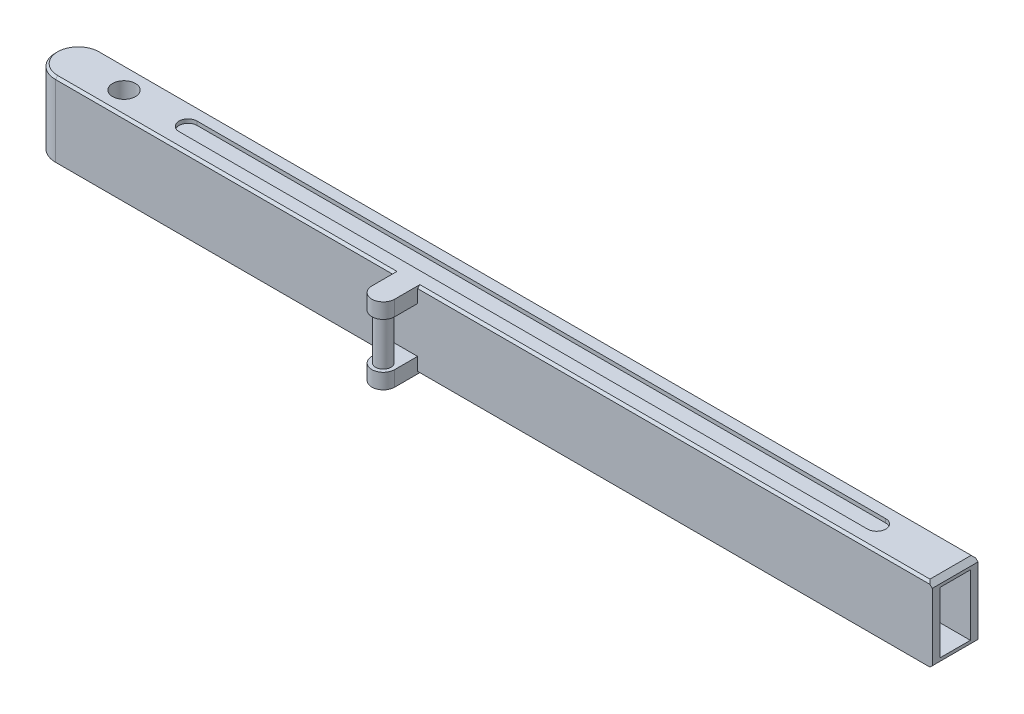
SolidWorks part; units mm, degrees
ref_plane "Front Plane" through (0, 0, 0) normal (0, 0, 1) x (1, 0, 0)
ref_plane "Top Plane" through (0, 0, 0) normal (0, 1, 0) x (1, 0, 0)
ref_plane "Right Plane" through (0, 0, 0) normal (1, 0, 0) x (0, 0, -1)
sketch "Sketch1" plane through (0, 0, 0) normal (0, 1, 0) x (1, 0, 0)
  line L0 (0, 0) -> (11500, 0)
  line L1 (11500, 0) -> (11500, 600)
  line L3 (0, 600) -> (694.445, 600)
  line L4 (11500, 300) -> (385.2625, 300) construction
  line L5 (11500, 600) -> (694.445, 600)
  arc A0 (0, 0) -> (0, 600) centre (0, 300) cw
  circle A2 centre (600, 300) radius 150
  dimension "D5" = 300
  dimension "D7" = 300
  dimension "D1" = 11500
  dimension "D2" = 600
  dimension "D3" = 90
  dimension "D8" = 10900
extrude "Boss-Extrude1" add sketch "Sketch1" along normal blind 1000
ref_plane "Plane1" through (0, 500, 0) normal (0, 1, 0) x (1, 0, 0)
sketch "Sketch3" plane through (0, 1000, 0) normal (0, 1, 0) x (1, 0, 0)
  line L0 (4600, 203.2624) -> (4600, -300) construction
  line L1 (4750, 203.2624) -> (4750, -300)
  line L2 (4450, 203.2624) -> (4450, -300)
  line L3 (-55, 0) -> (55, 0) construction
  arc A0 (4750, 203.2624) -> (4450, 203.2624) centre (4600, 203.2624) ccw
  arc A1 (4450, -300) -> (4750, -300) centre (4600, -300) ccw
  circle A2 centre (600, 300) radius 150 construction
  point P2 (4600, -48.3688)
  dimension "D1" = 150
  dimension "D3" = 4000
  dimension "D2" = 300
extrude "Boss-Extrude2" add sketch "Sketch3" against normal blind 200
mirror "Mirror1" about plane through (0, 500, 0) normal (0, 1, 0) of "Boss-Extrude2"
sketch "Sketch4" plane through (0, 800, 0) normal (0, -1, 0) x (1, 0, 0)
  circle A0 centre (4600, 300) radius 100
  dimension "D1" = 200
extrude "Boss-Extrude3" add sketch "Sketch4" along normal blind 700
sketch "Sketch5" plane through (11500, 0, 0) normal (1, 0, 0) x (0, 0, -1)
  line L0 (0, 55) -> (0, -55) construction
  line L1 (100, 900) -> (500, 900)
  line L2 (100, 900) -> (100, 100)
  line L3 (100, 100) -> (500, 100)
  line L4 (500, 900) -> (500, 100)
  line L5 (55, 0) -> (-55, 0) construction
  dimension "D1" = 400
  dimension "D2" = 100
  dimension "D3" = 800
  dimension "D4" = 100
extrude "Cut-Extrude1" cut sketch "Sketch5" against normal blind 10000
sketch "Sketch6" plane through (0, 0, 0) normal (0, -1, 0) x (1, 0, 0)
  line L0 (1432.066, -307.8009) -> (10462.7964, -307.8009) construction
  line L1 (1432.066, -188.6831) -> (10462.7964, -188.6831)
  line L2 (1432.066, -426.9188) -> (10462.7964, -426.9188)
  arc A0 (1432.066, -188.6831) -> (1432.066, -426.9188) centre (1432.066, -307.8009) ccw
  arc A1 (10462.7964, -426.9188) -> (10462.7964, -188.6831) centre (10462.7964, -307.8009) ccw
  point P2 (5947.4312, -307.8009)
extrude "Cut-Extrude2" cut sketch "Sketch6" against normal blind 50
mirror "Mirror2" about plane through (0, 500, 0) normal (0, 1, 0) of "Cut-Extrude2"
chamfer "Chamfer1" distance 30 angle 45 8 edges at (5750, 0, -600) (5750, 1000, -600) (-300, 0, -300) (-300, 1000, -300) (2225, 1000, 0) (2225, 0, 0) (8125, 0, 0) (8125, 1000, 0)
chamfer "Chamfer2" distance 60 angle 45 2 edges at (11500, 1000, -300) (11500, 0, -300)
